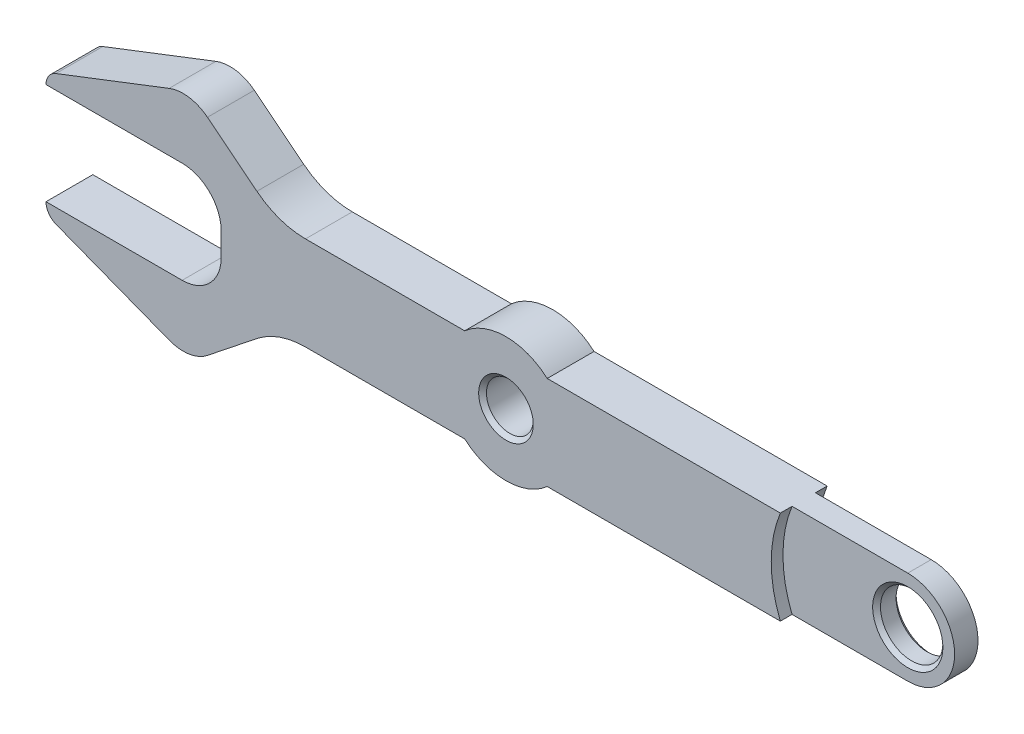
from build123d import *

# Parameters (mm, degrees)
BOSS_EXTRUDE1_DEPTH     = 3
SKETCH3_R               = 16
CUT_EXTRUDE1_DEPTH      = 1.5
CUT_EXTRUDE2_DEPTH      = 61.827729708
CUT_EXTRUDE2_DEPTH_BACK = 61.827729708
SKETCH4_R               = 4
SKETCH4_R_2             = 3
CHAMFER1_SIZE           = 0.5
FILLET1_R               = 10


with BuildPart() as part:
    # Sketch1 → Boss-Extrude1 (new, symmetric)
    with BuildSketch(Plane.XY):
        with BuildLine():
            Line((50, 6), (5.291502622, 6))
            ThreePointArc((5.291502622, 6), (0, 8), (-5.291502622, 6))
            Line((-5.291502622, 6), (-29.18544931, 6))
            Line((-29.18544931, 6), (-38.257859313, 13.216520767))
            ThreePointArc((-38.257859313, 13.216520767), (-40.615194579, 14.246112449), (-43.172428892, 13.967470655))
            Line((-43.172428892, 13.967470655), (-57.671397892, 8.365596269))
            ThreePointArc((-57.671397892, 8.365596269), (-58.600083665, 7.631017879), (-58.950599334, 6.5))
            Line((-58.950599334, 6.5), (-41.5, 6.5))
            ThreePointArc((-41.5, 6.5), (-37.964466094, 5.035533906), (-36.5, 1.5))
            Line((-36.5, 1.5), (-36.5, -1.5))
            ThreePointArc((-36.5, -1.5), (-37.964466094, -5.035533906), (-41.5, -6.5))
            Line((-41.5, -6.5), (-58.950599334, -6.5))
            ThreePointArc((-58.950599334, -6.5), (-58.600083665, -7.631017879), (-57.671397892, -8.365596269))
            Line((-57.671397892, -8.365596269), (-43.172428892, -13.967470655))
            ThreePointArc((-43.172428892, -13.967470655), (-40.615194579, -14.246112449), (-38.257859313, -13.216520767))
            Line((-38.257859313, -13.216520767), (-29.18544931, -6))
            Line((-29.18544931, -6), (-5.291502622, -6))
            ThreePointArc((-5.291502622, -6), (0, -8), (5.291502622, -6))
            Line((5.291502622, -6), (50, -6))
            ThreePointArc((50, -6), (56, 0), (50, 6))
        make_face()
    extrude(amount=BOSS_EXTRUDE1_DEPTH, both=True)

    # Sketch3 → Cut-Extrude1 (cut)
    with BuildSketch(Plane.XY.offset(3)):
        with Locations((50, 0)):
            Circle(SKETCH3_R)
    cut_extrude1 = extrude(amount=-CUT_EXTRUDE1_DEPTH, mode=Mode.SUBTRACT)

    # Mirror1: Cut-Extrude1 across plane
    add(cut_extrude1.mirror(Plane.XY), mode=Mode.SUBTRACT)

    # Sketch4 → Cut-Extrude2 (cut, two sides: drawn at the far end of the back side and taken through both)
    with BuildSketch(Plane.XY.offset(1.5).offset(-CUT_EXTRUDE2_DEPTH_BACK)):
        with Locations((50, 0)):
            Circle(SKETCH4_R)
        Circle(SKETCH4_R_2)
    extrude(amount=CUT_EXTRUDE2_DEPTH + CUT_EXTRUDE2_DEPTH_BACK, mode=Mode.SUBTRACT)

    # Chamfer1
    chamfer1_edges = [part.edges().sort_by_distance(p)[0] for p in [
        (46, 0, 1.5),
        (46, 0, -1.5),
        (-3, 0, -3),
        (-3, 0, 3),
    ]]
    chamfer(chamfer1_edges, length=CHAMFER1_SIZE)

    # Fillet1
    fillet1_edges = [part.edges().sort_by_distance(p)[0] for p in [
        (-29.18544931, 6, 0),
        (-29.18544931, -6, 0),
    ]]
    fillet(fillet1_edges, radius=FILLET1_R)


solid = part.part
